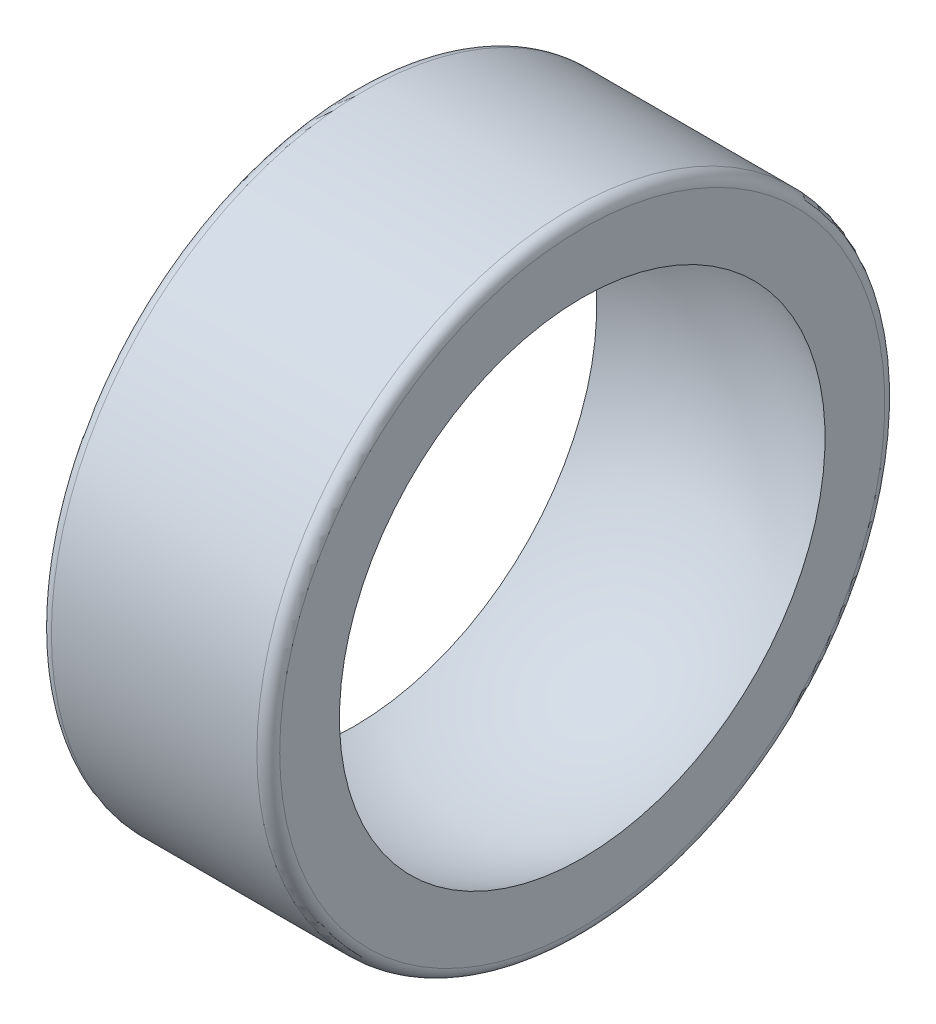
SolidWorks part; units mm, degrees
material "普通碳钢"
ref_plane "前视" through (0, 0, 0) normal (0, 0, 1) x (1, 0, 0)
ref_plane "上视" through (0, 0, 0) normal (0, 1, 0) x (1, 0, 0)
ref_plane "右视" through (0, 0, 0) normal (1, 0, 0) x (0, 0, -1)
sketch "草图1" plane through (0, 0, 0) normal (0, 0, 1) x (1, 0, 0)
  line L0 (-48.2313, 0) -> (54.1301, 0) construction
  line L1 (0, 38.2843) -> (0, -30.9976) construction
  line L2 (-10, 27.5) -> (-10, 21.2662)
  line L3 (10, 27.5) -> (10, 21.2662)
  line L4 (-10, 27.5) -> (10, 27.5)
  arc A0 (10, 21.2662) -> (-10, 21.2662) centre (0, 0) ccw
  dimension "D1" = 47
  dimension "D2" = 20
  dimension "D3" = 27.5
revolve "旋转1" add sketch "草图1" angle 360 about L0
fillet "圆角1" radius 1 2 edges at (10, 0, 27.5) (-10, 0, 27.5)
